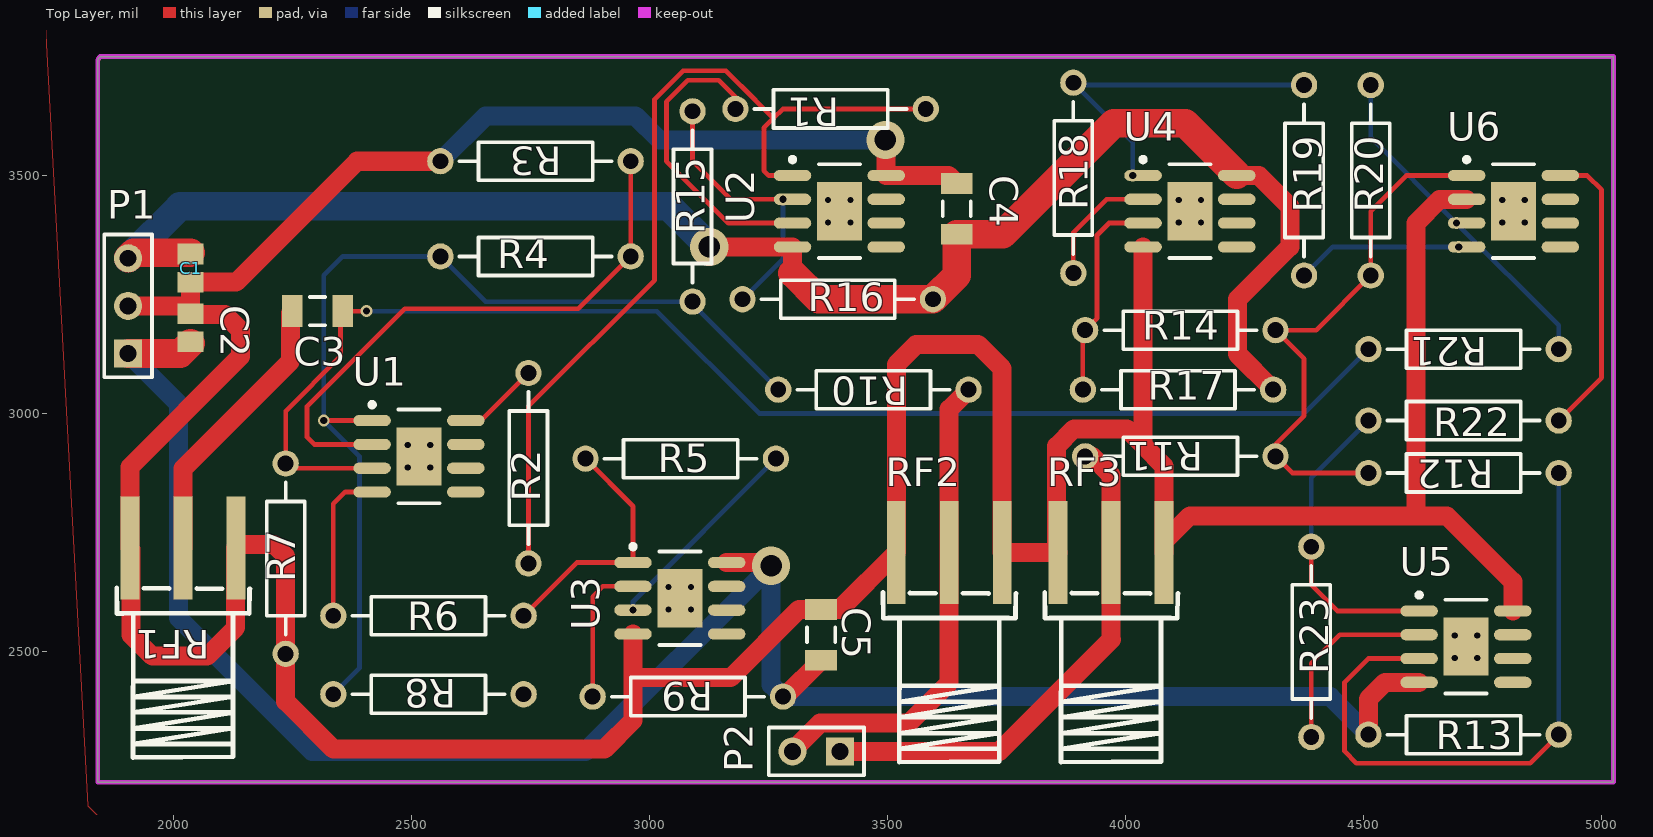
[diagram p0: Top Layer view]
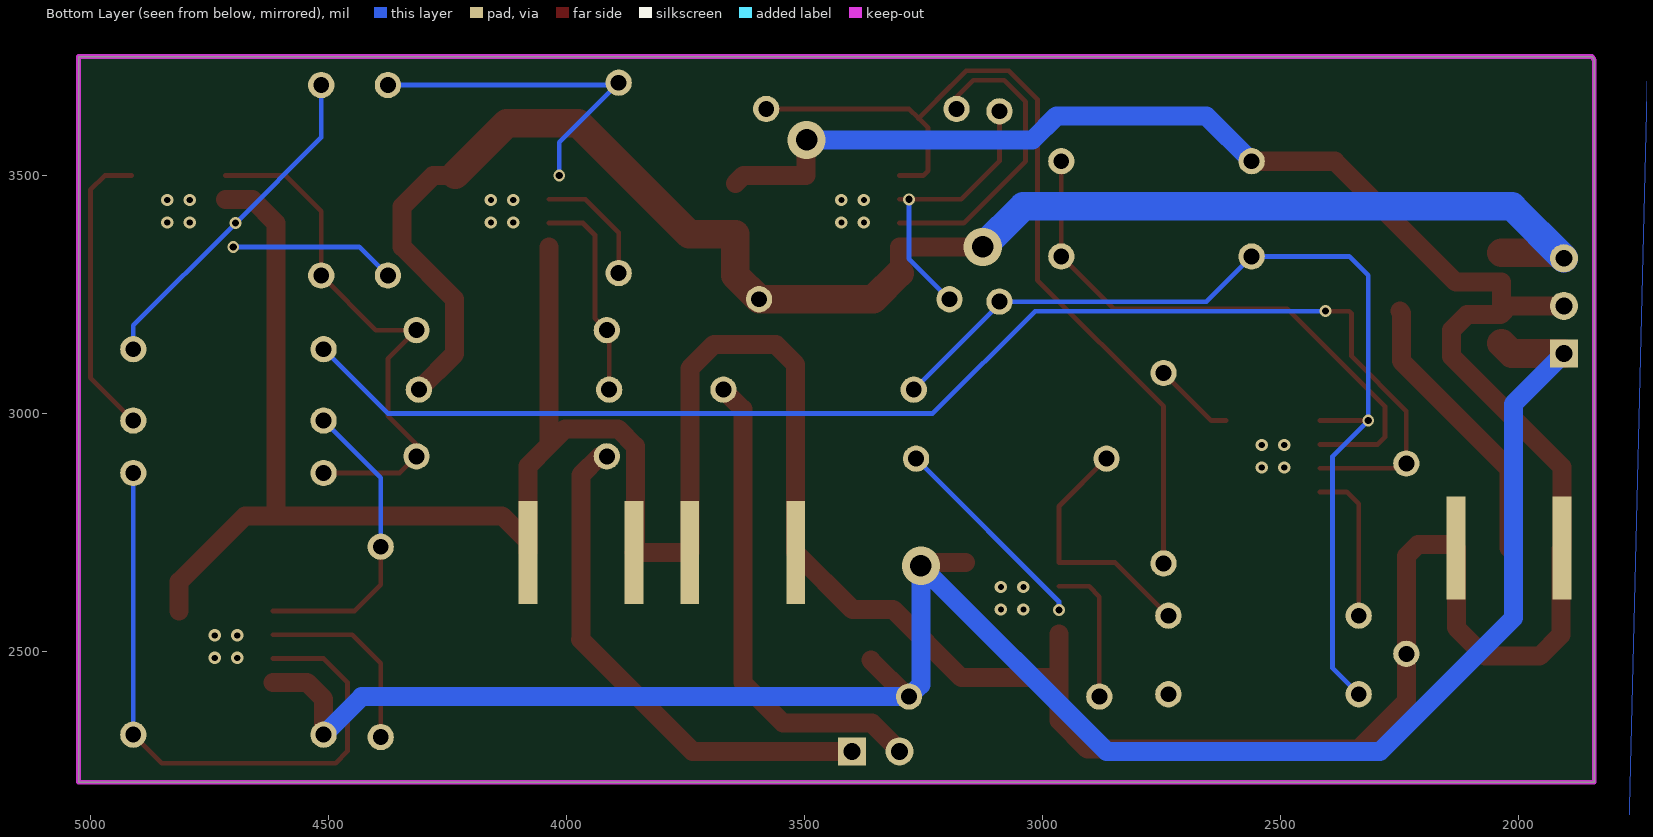
[diagram p1: Bottom Layer view, seen from below]
# Altium PCB MISC82821.PcbDoc
Units mil, origin at the board's own origin, x right, y up, seen from the top; angles counter-clockwise.
Board outline 3185 x 1525 mil, 2 copper layers (Top Layer, Bottom Layer); 39 components, 27 nets, 130 pads, 34 vias.
Unrouted connection lines stored in the file: 1.

## Layer stack, top to bottom (the 12.6 mil dielectric is the usual default, probably not edited)
Top Solder: solder mask 0.4, Solder Resist, Dk 3.5
Top Layer: signal copper 1.4
Dielectric 1: dielectric 12.6, FR-4, Dk 4.8
Bottom Layer: signal copper 1.4
Bottom Solder: solder mask 0.4, Solder Resist, Dk 3.5

## Board outline
1840,2225 5025,2225 5025,3750 1845,3750 ccw(c1857.07,3737.93) 1840,3737.93

## Design rules (kind name [scope] priority, off if disabled: settings)
AssemblyTestPointUsage [All] p0: scope1count=1 scope1_0_kind=Board scope1_0_value=Board scope2count=1 scope2_0_kind=Board scope2_0_value=Board commentlength=0
AssemblyTestpoint [All] p0: scope1count=1 scope1_0_kind=Board scope1_0_value=Board scope2count=1 scope2_0_kind=Board scope2_0_value=Board commentlength=0
Clearance [All] p0: scope1count=1 scope1_0_kind=Board scope1_0_value=Board scope2count=1 scope2_0_kind=Board scope2_0_value=Board commentlength=0 gap=10
Clearance [All] p1: gap=10
ComponentClearance [All] p0: scope1count=1 scope1_0_kind=Board scope1_0_value=Board scope2count=1 scope2_0_kind=Board scope2_0_value=Board commentlength=0 gap=10 collisioncheckmode=3
DiffPairsRouting [All] p0: scope1count=1 scope1_0_kind=Board scope1_0_value=Board scope2count=1 scope2_0_kind=Board scope2_0_value=Board commentlength=0
FabricationTestPointUsage [All] p0: scope1count=1 scope1_0_kind=Board scope1_0_value=Board scope2count=1 scope2_0_kind=Board scope2_0_value=Board commentlength=0 valid=0 allowmultiple=FALSE
FabricationTestpoint [All] p0: scope1count=1 scope1_0_kind=Board scope1_0_value=Board scope2count=1 scope2_0_kind=Board scope2_0_value=Board commentlength=0 side=3 testpointundercomponent=TRUE minsize=40 maxsize=100 preferedsize=60 minholesize=0 maxholesize=40 preferedholesize=32 testpointgrid=1
FanoutControl Fanout_Default [All] p0: scope1count=1 scope1_0_kind=Board scope1_0_value=Board scope2count=1 scope2_0_kind=Board scope2_0_value=Board commentlength=30 // Fanout_Default (Default Rule)
FanoutControl Fanout_Small [All] p0 off: scope1count=1 scope1_0_kind=Board scope1_0_value=Board scope2count=1 scope2_0_kind=Board scope2_0_value=Board commentlength=84 // Protel DXP Scope 1 Expression Was: (CompPinCount < 5)   Fanout_Small (Default Rule)
FanoutControl Fanout_SOIC [All] p0 off: scope1count=1 scope1_0_kind=Board scope1_0_value=Board scope2count=1 scope2_0_kind=Board scope2_0_value=Board commentlength=71 // Protel DXP Scope 1 Expression Was: IsSOIC   Fanout_SOIC (Default Rule)
FanoutControl Fanout_LCC [All] p0 off: scope1count=1 scope1_0_kind=Board scope1_0_value=Board scope2count=1 scope2_0_kind=Board scope2_0_value=Board commentlength=69 // Protel DXP Scope 1 Expression Was: IsLCC   Fanout_LCC (Default Rule)
FanoutControl Fanout_BGA [All] p0 off: scope1count=1 scope1_0_kind=Board scope1_0_value=Board scope2count=1 scope2_0_kind=Board scope2_0_value=Board commentlength=69 // Protel DXP Scope 1 Expression Was: IsBGA   Fanout_BGA (Default Rule)
Height [All] p0: scope1count=1 scope1_0_kind=Board scope1_0_value=Board scope2count=1 scope2_0_kind=Board scope2_0_value=Board commentlength=0
HoleSize [All] p0: scope1count=1 scope1_0_kind=Board scope1_0_value=Board scope2count=1 scope2_0_kind=Board scope2_0_value=Board commentlength=0 absolutevalues=TRUE maxlimit=100 minlimit=1 maxpercent=80.000 minpercent=20.000
HoleToHoleClearance [All] p0: scope1count=1 scope1_0_kind=Board scope1_0_value=Board scope2count=1 scope2_0_kind=Board scope2_0_value=Board commentlength=0
LayerPairs [All] p0: scope1count=1 scope1_0_kind=Board scope1_0_value=Board scope2count=1 scope2_0_kind=Board scope2_0_value=Board commentlength=0 enforce=TRUE
MinimumSolderMaskSliver [All] p0: scope1count=1 scope1_0_kind=Board scope1_0_value=Board scope2count=1 scope2_0_kind=Board scope2_0_value=Board commentlength=0
NetAntennae [All] p0: scope1count=1 scope1_0_kind=Board scope1_0_value=Board scope2count=1 scope2_0_kind=Board scope2_0_value=Board commentlength=0
PasteMaskExpansion [All] p0: scope1count=1 scope1_0_kind=Board scope1_0_value=Board scope2count=1 scope2_0_kind=Board scope2_0_value=Board commentlength=0 expansion=0
PlaneClearance [All] p0: scope1count=1 scope1_0_kind=Board scope1_0_value=Board scope2count=1 scope2_0_kind=Board scope2_0_value=Board commentlength=0 clearance=20
PlaneConnect [All] p0: scope1count=1 scope1_0_kind=Board scope1_0_value=Board scope2count=1 scope2_0_kind=Board scope2_0_value=Board commentlength=0 planeconnectstyle=Relief reliefexpansion=20 reliefentries=4 reliefconductorwidth=10 reliefairgap=10
PolygonConnect [All] p0: scope1count=1 scope1_0_kind=Board scope1_0_value=Board scope2count=1 scope2_0_kind=Board scope2_0_value=Board commentlength=0 connectstyle=Relief reliefconductorwidth=10 reliefentries=4 polygonreliefangle="90 Angle"
PolygonConnect [All] p1: connectstyle=Relief reliefconductorwidth=10 reliefentries=4 polygonreliefangle="90 Angle" airgapwidth=10
RoutingCorners [All] p0: scope1count=1 scope1_0_kind=Board scope1_0_value=Board scope2count=1 scope2_0_kind=Board scope2_0_value=Board commentlength=0 cornerstyle=45-Degree minsetback=100 maxsetback=100
RoutingLayers [All] p0: scope1count=1 scope1_0_kind=Board scope1_0_value=Board scope2count=1 scope2_0_kind=Board scope2_0_value=Board commentlength=0 top layer=Automatic bottom layer=Automatic
RoutingPriority [All] p0: scope1count=1 scope1_0_kind=Board scope1_0_value=Board scope2count=1 scope2_0_kind=Board scope2_0_value=Board commentlength=0
RoutingTopology [All] p0: scope1count=1 scope1_0_kind=Board scope1_0_value=Board scope2count=1 scope2_0_kind=Board scope2_0_value=Board commentlength=0 topology=Shortest
RoutingVias [All] p0: scope1count=1 scope1_0_kind=Board scope1_0_value=Board scope2count=1 scope2_0_kind=Board scope2_0_value=Board commentlength=0 holewidth=28 width=50 viastyle="Through Hole" minholewidth=28 minwidth=50 maxholewidth=28 maxwidth=50
RoutingVias [All] p1: holewidth=28 width=50 viastyle="Through Hole" minholewidth=28 minwidth=50 maxholewidth=28 maxwidth=50
ShortCircuit [All] p0: scope1count=1 scope1_0_kind=Board scope1_0_value=Board scope2count=1 scope2_0_kind=Board scope2_0_value=Board commentlength=0 allowed=FALSE
SilkToBoardRegionClearance [All] p0: scope1count=1 scope1_0_kind=Board scope1_0_value=Board scope2count=1 scope2_0_kind=Board scope2_0_value=Board commentlength=0
SilkToSilkClearance [All] p0: scope1count=1 scope1_0_kind=Board scope1_0_value=Board scope2count=1 scope2_0_kind=Board scope2_0_value=Board commentlength=0
SilkToSolderMaskClearance [All] p0 off: scope1count=1 scope1_0_kind=Board scope1_0_value=Board scope2count=1 scope2_0_kind=Board scope2_0_value=Board commentlength=44 // Protel DXP Scope 1 Expression Was: IsPad
SolderMaskExpansion [All] p0: scope1count=1 scope1_0_kind=Board scope1_0_value=Board scope2count=1 scope2_0_kind=Board scope2_0_value=Board commentlength=0 expansion=4
SolderMaskExpansion [All] p1: expansion=4
UnRoutedNet [All] p0: scope1count=1 scope1_0_kind=Board scope1_0_value=Board scope2count=1 scope2_0_kind=Board scope2_0_value=Board commentlength=0
UnpouredPolygon [All] p0: scope1count=1 scope1_0_kind=Board scope1_0_value=Board scope2count=1 scope2_0_kind=Board scope2_0_value=Board commentlength=0
Width [All] p0: scope1count=1 scope1_0_kind=Board scope1_0_value=Board scope2count=1 scope2_0_kind=Board scope2_0_value=Board commentlength=0 maxlimit=1000 minlimit=10 preferedwidth=10
Width [All] p1: maxlimit=1000 minlimit=10 preferedwidth=10 minimp=50.000000 maximp=50.000000 favimp=50.000000
30 further rules are at their usual default settings.

## Components (designator, comment, footprint, x,y, rotation, side; value= is the part's Value field where it differs from the comment)
C1 "100UF/100V" C0805 2035,3305.47 r270 top
C2 "100UF/100V" C0805 2035,3180 r270 top
C3 "104" C1206 2301.85,3215 r180 top
C4 "104" C1206 3645,3430 r270 top
C5 "104" C1206 3360,2535 r270 top
P1 "Header 3" HDR1X3 1903.94,3126.06 r90 top
P2 "Header 2" HDR1X2 3400,2290 r180 top
R1 "10K" AXIAL-0.4 3380,3640 r180 top
R2 "1" AXIAL-0.4 2745,2885 r270 top
R3 "10K" AXIAL-0.4 2760,3530 r0 top
R4 "51k" AXIAL-0.4 2760,3330 r180 top
R5 "10K" AXIAL-0.4 3065,2905 r0 top
R6 "1" AXIAL-0.4 2535,2575 r180 top
R7 "1K" AXIAL-0.4 2235,2695 r90 top
R8 "100K" AXIAL-0.4 2535,2410 r180 top
R9 "100K" AXIAL-0.4 3080,2405 r180 top
R10 "50" AXIAL-0.4 3470,3050 r180 top
R11 "50" AXIAL-0.4 4115,2910 r180 top
R12 "100K" AXIAL-0.4 4710,2875 r180 top
R13 "100K" AXIAL-0.4 4710,2325 r0 top
R14 "100K" AXIAL-0.4 4115,3175 r180 top
R15 "100K" AXIAL-0.4 3090,3435 r90 top
R16 "100K" AXIAL-0.4 3395,3240 r0 top
R17 "100K" AXIAL-0.4 4110,3050 r0 top
R18 "100K" AXIAL-0.4 3890,3495 r90 top
R19 "1" AXIAL-0.4 4375,3490 r90 top
R20 "51K" AXIAL-0.4 4515,3490 r90 top
R21 "10K" AXIAL-0.4 4710,3135 r180 top
R22 "1" AXIAL-0.4 4710,2985 r0 top
R23 "10K" AXIAL-0.4 4390,2520 r90 top
RF1 "SMA" SMA-SMD_HJ-SMA313 2020,2545 r0 top
RF2 "SMA" SMA-SMD_HJ-SMA313 3630,2535 r0 top
RF3 "SMA" SMA-SMD_HJ-SMA313 3970,2535 r0 top
U1 "LM7372MR" MRA08B_N 2515,2910 r0 top
U2 "LM7372MR" MRA08B_N 3398.43,3425 r0 top
U3 "LM7372MR" MRA08B_N 3063.23,2611.69 r0 top
U4 "LM7372MR" MRA08B_N 4135,3425 r0 top
U5 "LM7372MR" MRA08B_N 4715,2510 r0 top
U6 "LM7372MR" MRA08B_N 4815,3425 r0 top

## Footprints (in the part's own frame and the unit in brackets; to place one, negate y for a bottom-side part, rotate by r counter-clockwise, add the part's x,y. Pads: shape width x height; smd on the part's side, far side on the other; paste and mask are expansions set on the pad)
AXIAL-0.4 [mm] "Axial Device, Thru-Hole; 2 Leads; 0.4 in Pin Spacing"
  round 1.4 hole 0.85: 1(-5.08,0) 2(5.08,0)
  silkscreen extent -4.06,-1.02 4.06,1.02
C0805 [mm] "Chip Capacitor, Body 2.0x1.3mm, IPC High Density"
  rect 1.1x1.4 smd: 1(-0.75,0) 2(0.75,0)
C1206 [mm] "Chip Capacitor, Body 3.2x1.6mm, IPC High Density"
  rect 1.1x1.7 smd: 1(-1.35,0) 2(1.35,0)
  silkscreen extent -0.4,-0.75 0.4,0.75
HDR1X2 [mm] "Connector; Header; 2 Position"
  rect 1.5x1.5 hole 0.9: 1(0,0)
  round 1.5 hole 0.9: 2(2.54,0)
  silkscreen extent -1.27,-1.27 3.81,1.27
HDR1X3 [mm] "Connector; Header; 3 Position"
  rect 1.5x1.5 hole 0.9: 1(0,0)
  round 1.5 hole 0.9: 2(2.54,0) 3(5.08,0)
  silkscreen extent -1.27,-1.27 6.35,1.27
MRA08B_N [mm] "SOIC, 8-Leads, Body 4.9x3.9mm, Pitch 1.27mm, Exposed Pad, IPC Medium Density"
  oval 2x0.6 smd: 1(-2.5,1.905) 2(-2.5,0.635) 3(-2.5,-0.635) 4(-2.5,-1.905) 5(2.5,-1.905) 6(2.5,-0.635) 7(2.5,0.635) 8(2.5,1.905)
  rect 2.41x3.1 smd: 9(0,0)
  silkscreen extent -2.62,-2.5 1.1,2.88
SMA-SMD_HJ-SMA313 [mm]
  rect 1x5.5 smd paste+0 mask+0: 1(-0.02,4.379) 2(2.805,4.379) 3(-2.845,4.379)
  rect 1x5.5 smd far side paste+0 mask+0: 4(2.805,4.379) 5(-2.845,4.379)
  silkscreen extent -3.55,-6.8 3.55,2.26

## Part data
C1 C2: library part "Cap Pol3", "Polarized Capacitor (Surface Mount)"
C3 C4 C5: library part "Cap Semi", "Capacitor (Semiconductor SIM Model)"
P1: "Header, 3-Pin"
P2: "Header, 2-Pin"
R1 R2 R3 R4 R5 R6 R7 R8 R9 R10 R11 R12 R13 R14 R15 R16 R17 R18 R19 R20 R21 R22 R23: library part Res2, "Resistor"
RF1 RF3: library part SMB, "Antenna"
RF2: library part SMB, "TI antenna"
U1 U2 U3 U4 U5 U6: "High Speed, High Output Current, Dual Operational Amplifier, 9-pin PSOP"

## Via types
v1: diameter 25.98, hole 12.99, Top Layer to Bottom Layer, tented top, 24 vias
v2: diameter 25, hole 15, Top Layer to Bottom Layer, 7 vias
v3: diameter 80, hole 45, Top Layer to Bottom Layer, 3 vias

## Nets (pads, with @x,y where several pads share a name; then routed paths per layer and width w, separated by ;. In a path a pad name is that pad's centre, name@x,y a point inside that pad or via, vN(x,y) a via of type N, cw(c..) or ccw(c..) an arc to the next point about the centre after c; other vN are vias at no path point)
GND: C1.2 C2.1 C4.1 C5.1 P1.2 R3.1 R7.1 RF1.2 RF1.3 RF2.2 RF2.3 RF3.2 RF3.3 U2.8 U3.4 U4.4 U5.8 U6.2 | length 9270.2
  Top Layer w40: P1.2 2018.46,3226.06 C2.1 ; R3.1 2385,3530 2130.94,3275.94 C1.2 C2.1 ; U3.4 2965,2536.5 2965,2445 ; v3@3495,3560 3496.85,3558.15 U2.8 3628.15,3500 C4.1 ; U4.4 4036.57,2933.43 ; RF3.2 RF3.2@4080.43,2730.43 ; U6.2 4660,3450 4610,3400 4610,2785 ; U5.8 4813.43,2646.57 4675,2785 4610,2785 ; C2.1 2036.65,3207.87 2107.13,3207.87 2140,3175 2140,3120 1907.99,2887.99 RF1.3 1910,2715.39 1910,2535 1955,2490 2070,2490 2130,2550 2130,2716.97 RF1.2 2138.03,2725 2210,2725 2235,2700 R7.1 2235,2395 2335,2295 2905,2295 2965,2355 2965,2445 ; 2965,2445 3170,2445 3313.15,2588.15 C5.1 3398.74,2588.15 RF2.3 3517.99,3102.99 3560,3145 3690,3145 3740.43,3094.57 RF2.2 RF3.3 3855,2710.39 3855,2931.4 3891.16,2967.56 4002.44,2967.56 4036.57,2933.43 ; 4036.57,2933.43 4080.43,2889.57 RF3.2@4080.43,2730.43 ; RF3.2@4080.43,2730.43 4135,2785 4610,2785
  Bottom Layer w40: R3.1 2655,3625 2970,3625 3020,3575 v3(3495,3575)
NetC3_1: C3.1 R7.2 R21.2 U1.3 | length 2855.4
  Top Layer w10: v2(2405,3215) C3.1 2350,3210 2350,3120 2235,3005 R7.2 2245,2885 U1.3
  Bottom Layer w10: v2(2405,3215) 3015,3215 3230,3000 4375,3000 R21.2
NetP2_1: P2.1 R11.2 RF3.1 | length 1083.9
  Top Layer w40: P2.1 3735,2290 3970,2525 3969.21,2525.79 RF3.1 3969.21,2870.79 3930,2910 R11.2
NetP2_2: P2.2 R10.1 RF2.1 | length 1022.5
  Top Layer w40: P2.2 3300,2291.48 3358.05,2349.53 3369.38,2349.53 3369.85,2350 3545,2350 3629.21,2434.21 RF2.1 3629.21,3009.21 R10.1
NetR1_1: R1.1 R2.2 U2.1 | length 1911.9
  Top Layer w10: R2.2 2745,3015 3010,3280 3010,3660 3070,3720 3160.19,3720 3222.56,3657.63 3222.56,3657.44 3260,3620 ; U2.1 3250,3500 3240,3510 3240,3600 3260,3620 ; R1.1 3280,3640 3260,3620
NetR1_2: R1.2 U2.3 | length 647
  Top Layer w10: R1.2 3180,3665 3145,3700 3080,3700 3035,3655 3035,3530 3165,3400 U2.3
NetR2_1: R2.1 U1.8 | length 173
  Top Layer w10: U1.8 2645,2985 R2.1
NetR3_2: R3.2 R4.1 U1.2 | length 1218.3
  Top Layer w10: U1.2 2295,2935 2280,2950 2280,3015 2485,3220 2850,3220 R4.1 R3.2
NetR4_2: R4.2 R8.2 R10.2 R15.1 U1.1 | length 2123
  Top Layer w10: v2(2315,2985) U1.1
  Bottom Layer w10: R8.2 2390,2465 2390,2910 v2(2315,2985) 2315,3290 2355,3330 R4.2 2655,3235 3085,3235 R10.2
NetR5_1: R5.1 R6.1 U3.1 | length 535.7
  Top Layer w10: R6.1 2846.69,2686.69 U3.1 2964.8,2805.2 R5.1
NetR5_2: R5.2 U3.3 | length 442.7
  Bottom Layer w10: v2(2964.8,2586.69) 2964.8,2604.8 R5.2
NetR6_2: R6.2 U1.4 | length 326.9
  Top Layer w10: R6.2 2335,2810 2360,2835 U1.4
NetR8_1: R8.1 R9.2 U3.2 | length 303.8
  Top Layer w10: R9.2 2880,2615 2901.69,2636.69 U3.2
NetR11_1: R11.1 R12.2 R14.1 R20.1 U6.1 | length 1139.5
  Top Layer w10: R12.2 4350,2875 R11.1 4315,2935 4375,2995 4375,3115 R14.1 4400,3175 R20.1 4515,3425 4590,3500 U6.1
NetR12_1: R12.1 R13.2 U5.3 | length 1357.5
  Top Layer w10: U5.3 4510,2485 4460,2435 4460,2290 4485,2265 4850,2265 R13.2
  Bottom Layer w10: R13.2 R12.1
NetR14_2: R14.2 R17.1 U4.3 | length 444.4
  Top Layer w10: R17.1 3910,3170 R14.2 3940,3200 3940,3375 3965,3400 U4.3
NetR15_2: R15.2 R16.1 U2.2 | length 613.3
  Top Layer w10: R15.2@3070,3635 R15.2 3090,3530 3170,3450 v2(3280,3450) U2.2
  Bottom Layer w10: R16.1 3280,3325 v2(3280,3450)
NetR18_1: R18.1 U4.2 | length 260.6
  Top Layer w10: R18.1 3890,3380 3960,3450 U4.2
NetR18_2: R18.2 R19.2 U4.1 | length 726.8
  Bottom Layer w10: R18.2 R18.2@3895,3690 ; v2(4015,3500) 4015,3570 R18.2@3895,3690 ; R19.2 R18.2@3895,3690
NetR19_1: R19.1 U6.4 | length 349.9
  Bottom Layer w10: R19.1 4435,3350 v2(4700,3350)
NetR20_2: R20.2 R21.1 U6.3 | length 718.6
  Bottom Layer w10: R20.2 4515,3580 v2(4695,3400) 4910,3185 R21.1
NetR22_1: R22.1 R23.2 U5.1 | length 644.1
  Top Layer w10: R23.2 4390,2640 4445,2585 U5.1
  Bottom Layer w10: R23.2 4390,2865 R22.1
NetR22_2: R22.2 U6.8 | length 621.3
  Top Layer w10: R22.2 5000,3075 5000,3470 4970,3500 U6.8
NetR23_1: R23.1 U5.2 | length 406.4
  Top Layer w10: R23.1 4390,2475 4450,2535 U5.2
VCC: C1.1 C4.2 P1.3 R16.2 R17.2 U2.4 U4.8 | length 3472.5
  Top Layer w40: v3(3125,3350) U2.4 3300,3295 ; U4.8 4280,3500 4345,3435 4345,3350 4235,3240 4235,3125 R17.2
  Top Layer w60: P1.3 1915.47,3337.6 C1.1@2035,3337.6 ; 3300,3295 3355,3240 R16.2 3645,3290 C4.2 3741.85,3376.85 3975,3610 4125,3610 4233.19,3501.81 U4.8@4233.43,3501.81
  Bottom Layer w60: P1.3 2012.87,3435 3040,3435 v3(3125,3350)
VEE: C2.2 C5.2 P1.1 R9.1 R13.1 U3.8 U5.4 | length 4215.1
  Top Layer w40: U3.8 3248.31,2686.69 v3(3255,2680) ; R9.1 3283.15,2405 C5.2 ; R13.1 4510,2400 4545,2435 U5.4
  Top Layer w60: P1.1 2013.19,3126.06 C2.2@2035,3147.87
  Bottom Layer w40: P1.1 2010,3020 2010,2570 2290,2290 2865,2290 v3(3255,2680) 3255,2430 R9.1 4430,2405 R13.1
VIN: C3.2 RF1.1 | length 592.7
  Top Layer w40: RF1.1 2019.21,2884.21 2245,3110 2245,3211.3 C3.2
pads on no net: RF1.4 RF1.5 RF2.4 RF2.5 RF3.4 RF3.5 U1.5 U1.6 U1.7 U1.9 U2.5 U2.6 U2.7 U2.9 U3.5 U3.6 U3.7 U3.9 U4.5 U4.6 U4.7 U4.9 U5.5 U5.6 U5.7 U5.9 U6.5 U6.6 U6.7 U6.9
copper on no net:
  other v1: 4691.38,2486.38 4738.62,2486.38 4691.38,2533.62 4738.62,2533.62 3039.61,2588.07 3086.85,2588.07 3039.61,2635.31 3086.85,2635.31 2491.38,2886.38 2538.62,2886.38 2491.38,2933.62 2538.62,2933.62 3374.8,3401.38 3422.05,3401.38 4111.38,3401.38 4158.62,3401.38 4791.38,3401.38 4838.62,3401.38 3374.8,3448.62 3422.05,3448.62 4111.38,3448.62 4158.62,3448.62 4791.38,3448.62 4838.62,3448.62

## Polygon pours and split planes (outlines as drawn)
GND on Bottom Layer "Top Layer-No Net" (solid, remove dead copper, pour order 4): 1725,3850 1755,3880 5120,3880 5120,2050 5170,2000 1770,2000
GND on Top Layer "Top Layer-No Net" (solid, remove dead copper, pour order 6): 1720,3990 5205,3990 5205,1770 2225,1770 1820,2175

## Keep-outs
Keep-Out Layer:
  lines w10: 1840,2225 1840,3737.93 cw(c1857.07,3737.93) 1845,3750 5025,3750 5025,2225 1850,2225 1840,2225